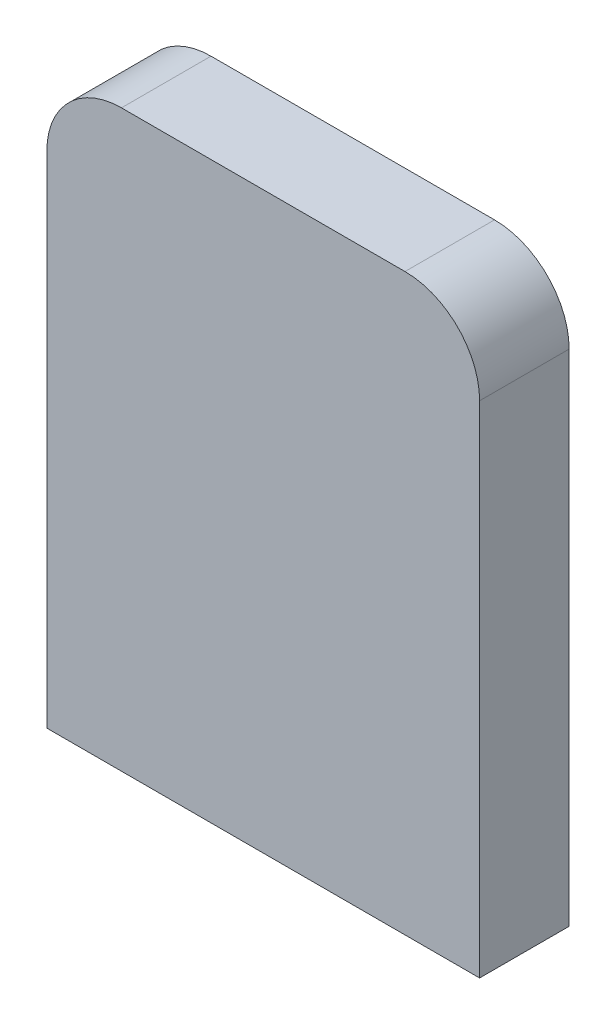
SolidWorks part; units mm, degrees
material "AISI 1045 钢，冷拔"
ref_plane "Front Plane" through (0, 0, 0) normal (0, 0, 1) x (1, 0, 0)
ref_plane "Top Plane" through (0, 0, 0) normal (0, 1, 0) x (1, 0, 0)
ref_plane "Right Plane" through (0, 0, 0) normal (1, 0, 0) x (0, 0, -1)
sketch "Sketch1" plane through (0, 0, 0) normal (0, 0, 1) x (1, 0, 0)
  line L1 (-29, -38.5) -> (29, -38.5)
  line L2 (-29, -38.5) -> (-29, 38.5)
  line L3 (-29, 38.5) -> (29, 38.5)
  line L4 (29, -38.5) -> (29, 38.5)
  line L5 (-29, -38.5) -> (29, 38.5) construction
  line L6 (-29, 38.5) -> (29, -38.5) construction
  point P0 (0, 0)
  dimension "D1" = 58
  dimension "D2" = 77
extrude "Boss-Extrude1" add sketch "Sketch1" along normal blind 12
fillet "Fillet1" radius 10 2 edges at (-29, 38.5, 6) (29, 38.5, 6)
sketch "Sketch2" plane through (0, 0, 12) normal (0, 0, 1) x (1, 0, 0)
  line L1 (19, 38.5) -> (-19, 38.5) construction
  point P1 (0, 28.5)
  point P5 (0, 38.5)
  dimension "D1" = 10
